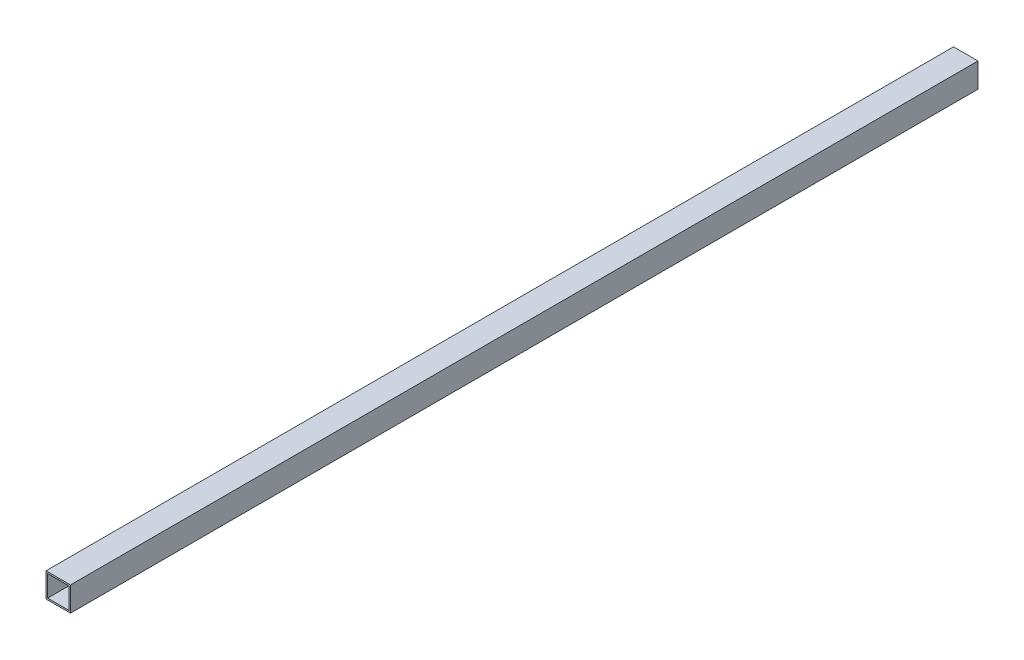
from build123d import *

# Parameters (mm, degrees)
SKETCH_1_W      = 30
SKETCH_1_H      = 30
SKETCH_1_W_2    = 26
SKETCH_1_H_2    = 26
EXTRUDE_1_DEPTH = 556


with BuildPart() as part:
    # 草图1 → 凸台-拉伸1 (new, symmetric)
    with BuildSketch(Plane.XY):
        Rectangle(SKETCH_1_W, SKETCH_1_H)
        Rectangle(SKETCH_1_W_2, SKETCH_1_H_2, mode=Mode.SUBTRACT)
    extrude(amount=EXTRUDE_1_DEPTH, both=True)


solid = part.part
